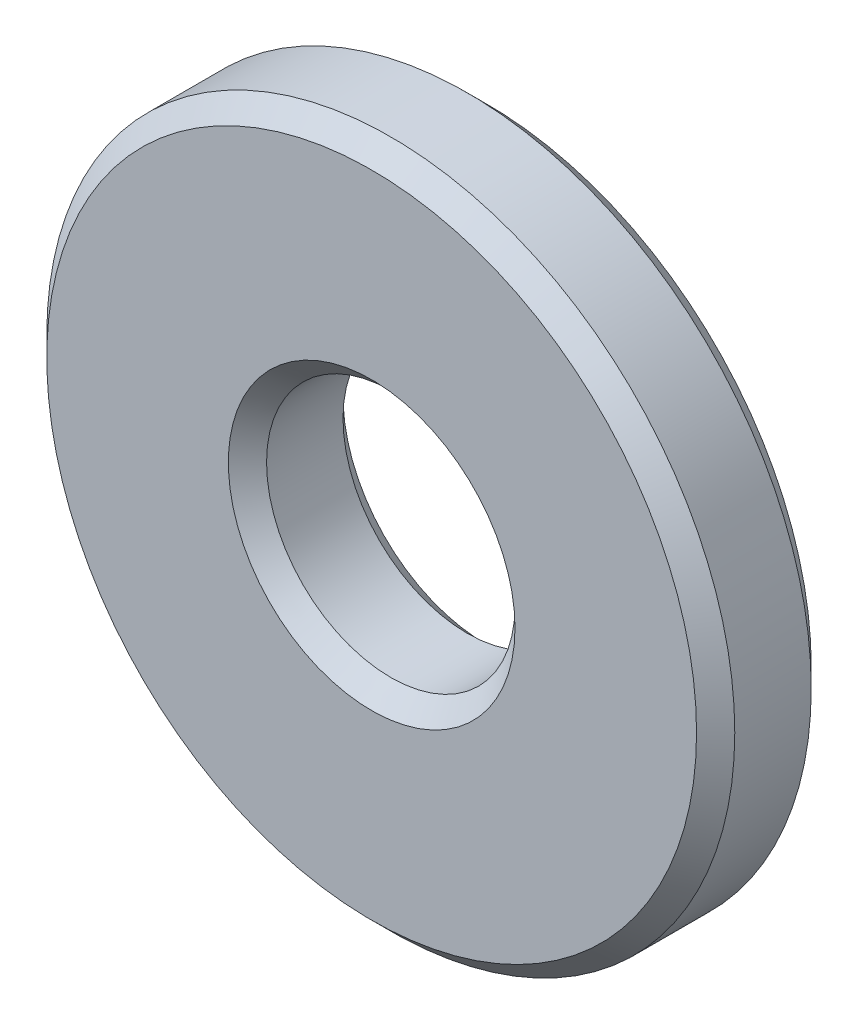
from build123d import *

# Parameters (mm, degrees)
SKETCH1_R           = 9
SKETCH1_R_2         = 3.25
BOSS_EXTRUDE1_DEPTH = 3
CHAMFER1_SIZE       = 0.5


with BuildPart() as part:
    # Sketch1 → Boss-Extrude1 (new body)
    with BuildSketch(Plane.XY):
        Circle(SKETCH1_R)
        Circle(SKETCH1_R_2, mode=Mode.SUBTRACT)
    extrude(amount=BOSS_EXTRUDE1_DEPTH)

    # Chamfer1
    chamfer1_edges = [part.edges().sort_by_distance(p)[0] for p in [
        (-9, 0, 0),
        (-9, 0, 3),
        (-3.25, 0, 0),
        (-3.25, 0, 3),
    ]]
    chamfer(chamfer1_edges, length=CHAMFER1_SIZE)


solid = part.part
